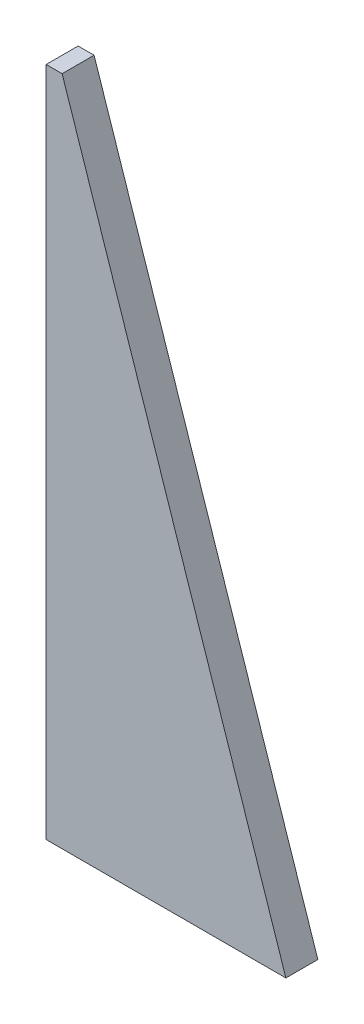
SolidWorks part; units mm, degrees
material "Q235B"
ref_plane "Front Plane" through (0, 0, 0) normal (0, 0, 1) x (1, 0, 0)
ref_plane "Top Plane" through (0, 0, 0) normal (0, 1, 0) x (1, 0, 0)
ref_plane "Right Plane" through (0, 0, 0) normal (1, 0, 0) x (0, 0, -1)
sketch "Sketch1" plane through (0, 0, 0) normal (0, 0, 1) x (1, 0, 0)
  line L0 (0, 0) -> (150, 0)
  line L1 (0, 0) -> (0, 420)
  line L2 (10, 420) -> (150, 0)
  line L3 (0, 420) -> (10, 420)
  dimension "D1" = 150
  dimension "D2" = 420
  dimension "D3" = 10
extrude "Boss-Extrude1" add sketch "Sketch1" along normal blind 20
